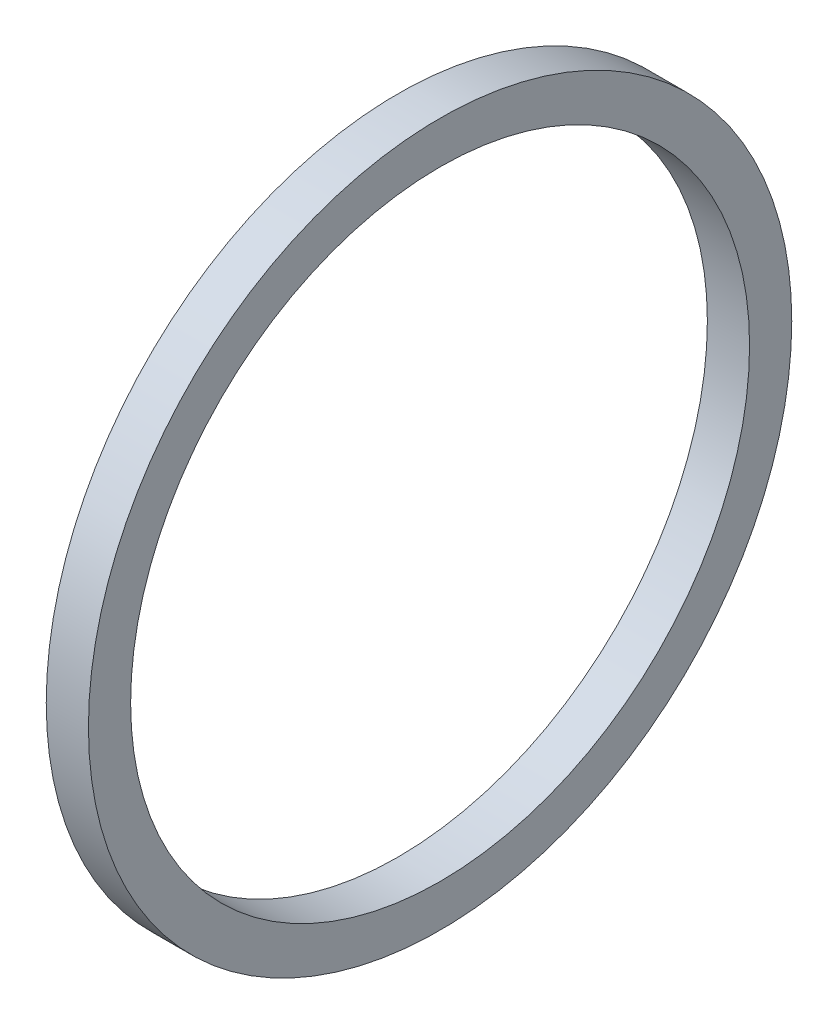
SolidWorks part; units mm, degrees
ref_plane "Front Plane" through (0, 0, 0) normal (0, 0, 1) x (1, 0, 0)
ref_plane "Top Plane" through (0, 0, 0) normal (0, 1, 0) x (1, 0, 0)
ref_plane "Right Plane" through (0, 0, 0) normal (1, 0, 0) x (0, 0, -1)
other "Configuration Table"
sketch "Sketch1" plane through (0, 0, 0) normal (0, 0, 1) x (1, 0, 0)
  line L0 (0, 0) -> (-50, 0)
  line L1 (-50, 48.55) -> (-50, 50)
  line L2 (-50, 50) -> (-44, 50)
  line L3 (-44, 50) -> (-44, 44)
  line L4 (-44, 44) -> (-50, 44)
  line L5 (-50, 44) -> (-50, 46)
  line L6 (-50, 46) -> (-45.5, 46)
  line L7 (-45.5, 46) -> (-45.5, 48.55)
  line L8 (-45.5, 48.55) -> (-50, 48.55)
  dimension "D1" = 50
  dimension "D2" = 6
  dimension "D3" = 1.45
  dimension "D4" = 2
  dimension "D5" = 6
  dimension "D6" = 4.5
  dimension "D7" = 44
revolve "Revolve1" add sketch "Sketch1" angle 360 about L0
